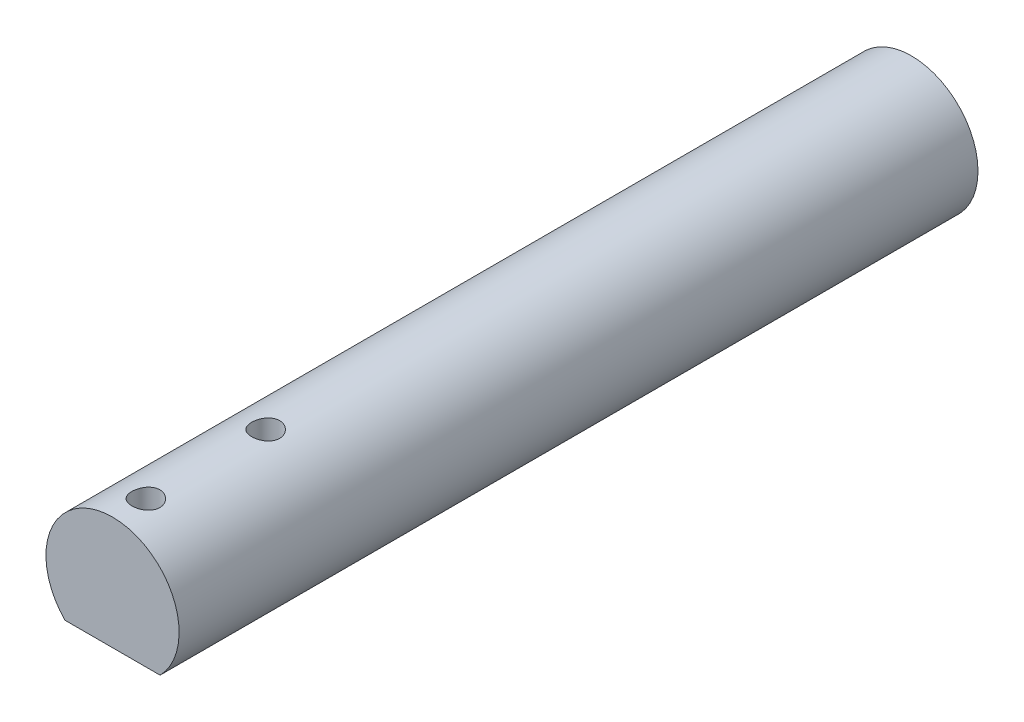
from build123d import *

# Parameters (mm, degrees)
SKETCH_1_R             = 10
EXTRUDE_1_DEPTH        = 60
HOLE_WIZARD_M6_1_D     = 5
HOLE_WIZARD_M6_1_DEPTH = 15
HOLE_WIZARD_M6_1_TIP   = 1.502151548
SKETCH_5_W             = 14.282856858
SKETCH_5_H             = 6
CUT_EXTRUDE_1_DEPTH    = 30
HOLE_WIZARD_M5_1_D     = 4.2


with BuildPart() as part:
    # 草图1 → 凸台-拉伸1 (new, symmetric)
    with BuildSketch(Plane.XY):
        Circle(SKETCH_1_R)
    extrude(amount=EXTRUDE_1_DEPTH, both=True)

    # M6 螺纹孔1
    with Locations(Plane(origin=(0, 0, -60), x_dir=(-1, 0, 0), z_dir=(0, 0, -1))):
        with Locations((0, 0)):
            Hole(HOLE_WIZARD_M6_1_D / 2, depth=HOLE_WIZARD_M6_1_DEPTH)
            with Locations((0, 0, -(HOLE_WIZARD_M6_1_DEPTH + HOLE_WIZARD_M6_1_TIP / 2))):  # 118° drill point
                Cone(0, HOLE_WIZARD_M6_1_D / 2, HOLE_WIZARD_M6_1_TIP, mode=Mode.SUBTRACT)

    # 草图5 → 切除-拉伸1 (cut)
    with BuildSketch(Plane.XY.offset(60)):
        with Locations((0, -10)):
            Rectangle(SKETCH_5_W, SKETCH_5_H)
    extrude(amount=-CUT_EXTRUDE_1_DEPTH, mode=Mode.SUBTRACT)

    # M5 螺纹孔1 (through all)
    with Locations(Plane(origin=(0, -7, 0), x_dir=(-1, 0, 0), z_dir=(0, -1, 0))):
        with Locations((0, -55), (0, -37)):
            Hole(HOLE_WIZARD_M5_1_D / 2)


solid = part.part
